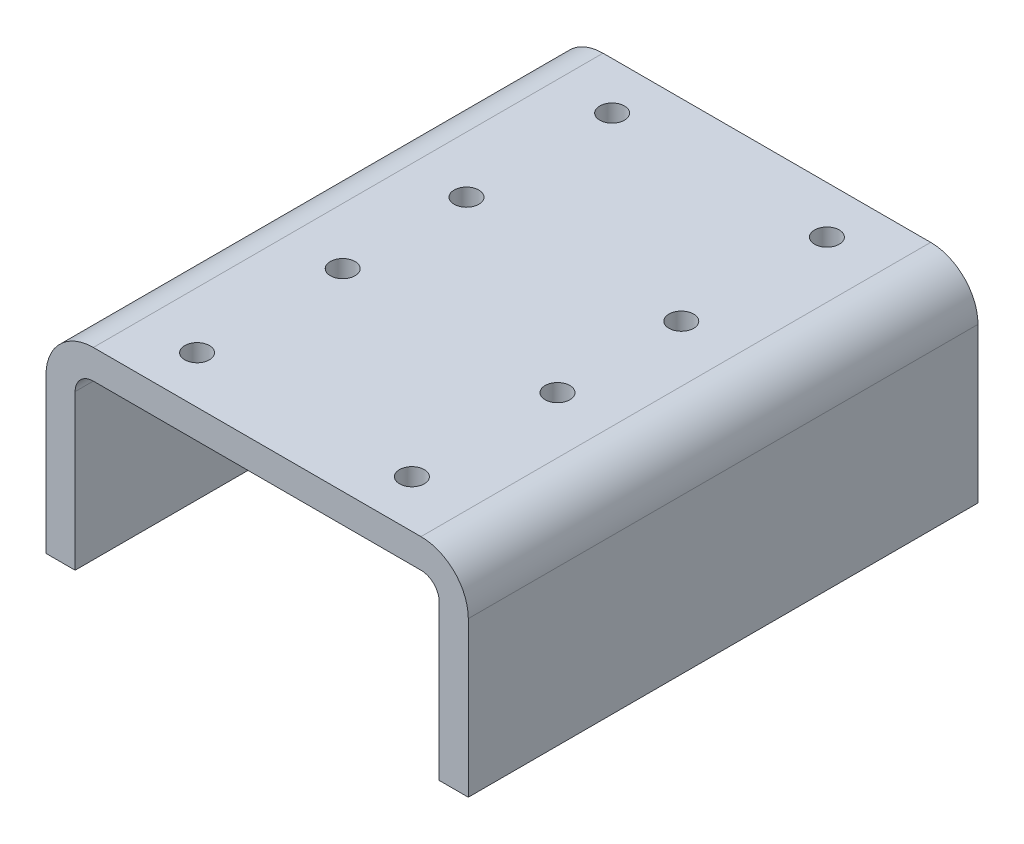
SolidWorks part; units mm, degrees
material "1023 carbon steel plate (SS)"
ref_plane "Front Plane" through (0, 0, 0) normal (0, 0, 1) x (1, 0, 0)
ref_plane "Top Plane" through (0, 0, 0) normal (0, 1, 0) x (1, 0, 0)
ref_plane "Right Plane" through (0, 0, 0) normal (1, 0, 0) x (0, 0, -1)
sketch "Sketch1" plane through (0, 0, 0) normal (0, 0, 1) x (1, 0, 0)
  line L0 (0, 0) -> (0, 42.5)
  line L1 (13, 55.5) -> (103, 55.5)
  line L2 (116, 42.5) -> (116, 0)
  line L3 (8, 0) -> (8, 42.5)
  line L4 (13, 47.5) -> (103, 47.5)
  line L5 (108, 42.5) -> (108, 0)
  line L6 (8, 0) -> (0, 0)
  line L7 (116, 0) -> (108, 0)
  arc A0 (103, 55.5) -> (116, 42.5) centre (103, 42.5) cw
  arc A1 (0, 42.5) -> (13, 55.5) centre (13, 42.5) cw
  arc A2 (8, 42.5) -> (13, 47.5) centre (13, 42.5) cw
  arc A3 (103, 47.5) -> (108, 42.5) centre (103, 42.5) cw
  point P7 (116, 55.5)
  point P10 (0, 55.5)
  dimension "D4" = 13
  dimension "D1" = 55.5
  dimension "D2" = 116
  dimension "D3" = 55.5
  dimension "D5" = 8
extrude "Boss-Extrude1" add sketch "Sketch1" along normal blind 140 contours L7 L5 A3 L4 A2 L3 L6 L0 A1 L1 A0 L2
sketch "Sketch2" plane through (0, 55.5, 0) normal (0, 1, 0) x (1, 0, 0)
  line L0 (0, -140) -> (0, 0) construction
  line L1 (13, -140) -> (103, -140) construction
  circle A0 centre (28.5, -13) radius 3
  circle A1 centre (87.5, -13) radius 3
  circle A2 centre (28.5, -53) radius 3
  circle A3 centre (87.5, -53) radius 3
  circle A4 centre (28.5, -87) radius 3
  circle A5 centre (87.5, -87) radius 3
  circle A6 centre (28.5, -127) radius 3
  circle A7 centre (87.5, -127) radius 3
  dimension "D2" = 28.5
  dimension "D3" = 40
  dimension "D5" = 40
  dimension "D6" = 34
  dimension "D7" = 6
  dimension "D1" = 59
  dimension "D4" = 13
hole_wizard "M8 Tapped Hole1" positions "Sketch3" profile "Sketch4" tap size "M8" standard "ISO"
sketch "Sketch3" plane through (0, 55.5, 0) normal (0, 1, 0) x (1, 0, 0)
  point P0 (28.5, -13)
  point P3 (87.5, -13)
  point P6 (87.5, -53)
  point P9 (28.5, -53)
  point P12 (28.5, -87)
  point P15 (87.5, -87)
  point P18 (87.5, -127)
  point P21 (28.5, -127)
sketch "Sketch4" plane through (28.5, 55.5, 13) normal (1, 0, 0) x (0, 0, 1)
  line L0 (0, 0) -> (0, 21.7929)
  line L1 (0, 21.7929) -> (3.4, 19.75)
  line L2 (3.4, 19.75) -> (3.4, 0)
  line L5 (3.4, 0) -> (0, 0)
  line L10 (0, 21.7929) -> (-3.4, 19.75) construction
  line L11 (0, -6.35) -> (0, 107.95) construction
  dimension "螺纹孔钻头直径" = 6.8
  dimension "螺纹孔钻头深度" = 19.75
  dimension "导头角度" = 118
cosmetic thread "Cosmetic thread 1"
cosmetic thread "Cosmetic thread 2"
cosmetic thread "Cosmetic thread 3"
cosmetic thread "Cosmetic thread 4"
cosmetic thread "Cosmetic thread 5"
cosmetic thread "Cosmetic thread 6"
cosmetic thread "Cosmetic thread 7"
cosmetic thread "Cosmetic thread 8"
